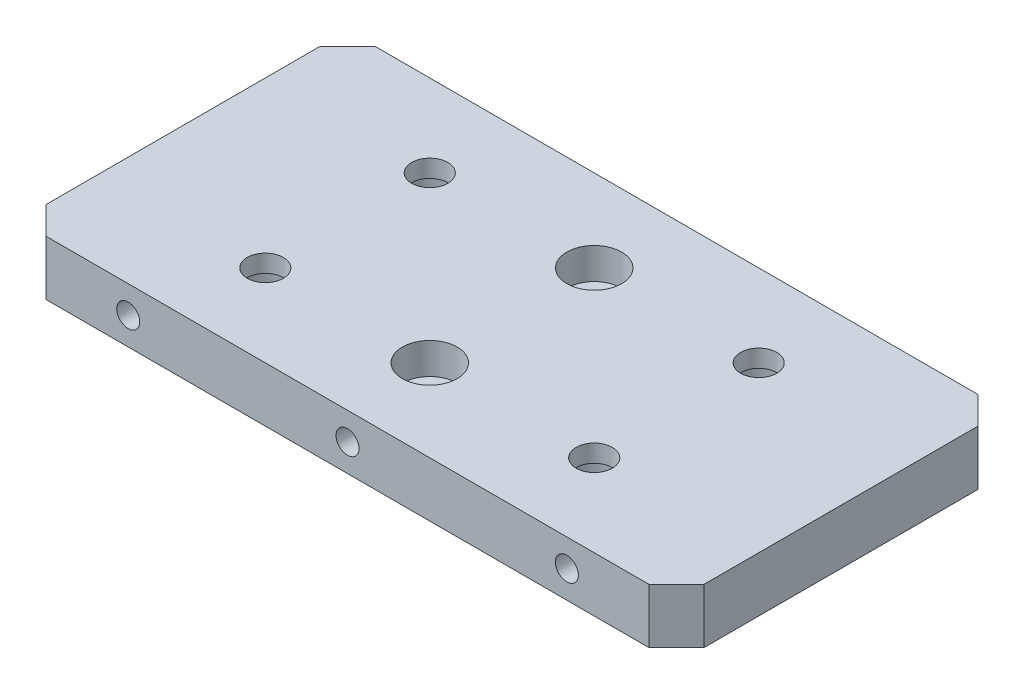
from build123d import *

# Parameters (mm, degrees)
SKETCH_1_W                = 120
SKETCH_1_H                = 60
EXTRUDE_1_DEPTH           = 10
CHAMFER_1_SIZE            = 5
HOLE_WIZARD_M5_1_D        = 4.2
HOLE_WIZARD_M5_1_DEPTH    = 12.4
HOLE_WIZARD_M5_1_TIP      = 1.2618073
HOLE_WIZARD_1_D           = 6.6
HOLE_WIZARD_1_DEPTH       = 12.4
HOLE_WIZARD_1_CBORE_D     = 11
HOLE_WIZARD_1_CBORE_DEPTH = 6.8
HOLE_WIZARD_1_TIP         = 1.982840043
HOLE_WIZARD_2_D           = 5.5
HOLE_WIZARD_2_DEPTH       = 12.4
HOLE_WIZARD_2_CBORE_D     = 10
HOLE_WIZARD_2_CBORE_DEPTH = 5.7
HOLE_WIZARD_2_TIP         = 1.652366702


with BuildPart() as part:
    # 草图1 → 凸台-拉伸1 (new body)
    with BuildSketch(Plane(origin=(0, 0, 0), x_dir=(1, 0, 0), z_dir=(0, 1, 0))):
        Rectangle(SKETCH_1_W, SKETCH_1_H)
    extrude(amount=EXTRUDE_1_DEPTH)

    # 倒角1
    chamfer_1_edges = [part.edges().sort_by_distance(p)[0] for p in [
        (60, 5, 30),
        (-60, 5, 30),
        (-60, 5, -30),
        (60, 5, -30),
    ]]
    chamfer(chamfer_1_edges, length=CHAMFER_1_SIZE)

    # M5 螺纹孔1
    with Locations(Plane.XY.offset(30)):
        with Locations((-40, 5), (0, 5), (40, 5)):
            Hole(HOLE_WIZARD_M5_1_D / 2, depth=HOLE_WIZARD_M5_1_DEPTH)
            with Locations((0, 0, -(HOLE_WIZARD_M5_1_DEPTH + HOLE_WIZARD_M5_1_TIP / 2))):  # 118° drill point
                Cone(0, HOLE_WIZARD_M5_1_D / 2, HOLE_WIZARD_M5_1_TIP, mode=Mode.SUBTRACT)

    # 打孔尺寸(%根据)内六角圆柱头螺钉的类型1
    with Locations(Plane(origin=(0, 0, 0), x_dir=(-1, 0, 0), z_dir=(0, -1, 0))):
        with Locations((30, -15), (30, 15), (-30, -15), (-30, 15)):
            CounterBoreHole(HOLE_WIZARD_1_D / 2, HOLE_WIZARD_1_CBORE_D / 2, HOLE_WIZARD_1_CBORE_DEPTH, depth=HOLE_WIZARD_1_DEPTH)
            with Locations((0, 0, -(HOLE_WIZARD_1_DEPTH + HOLE_WIZARD_1_TIP / 2))):  # 118° drill point
                Cone(0, HOLE_WIZARD_1_D / 2, HOLE_WIZARD_1_TIP, mode=Mode.SUBTRACT)

    # 打孔尺寸(%根据)内六角圆柱头螺钉的类型2
    with Locations(Plane(origin=(0, 10, 0), x_dir=(1, 0, 0), z_dir=(0, 1, 0))):
        with Locations((0, -15), (0, 15)):
            CounterBoreHole(HOLE_WIZARD_2_D / 2, HOLE_WIZARD_2_CBORE_D / 2, HOLE_WIZARD_2_CBORE_DEPTH, depth=HOLE_WIZARD_2_DEPTH)
            with Locations((0, 0, -(HOLE_WIZARD_2_DEPTH + HOLE_WIZARD_2_TIP / 2))):  # 118° drill point
                Cone(0, HOLE_WIZARD_2_D / 2, HOLE_WIZARD_2_TIP, mode=Mode.SUBTRACT)


solid = part.part
